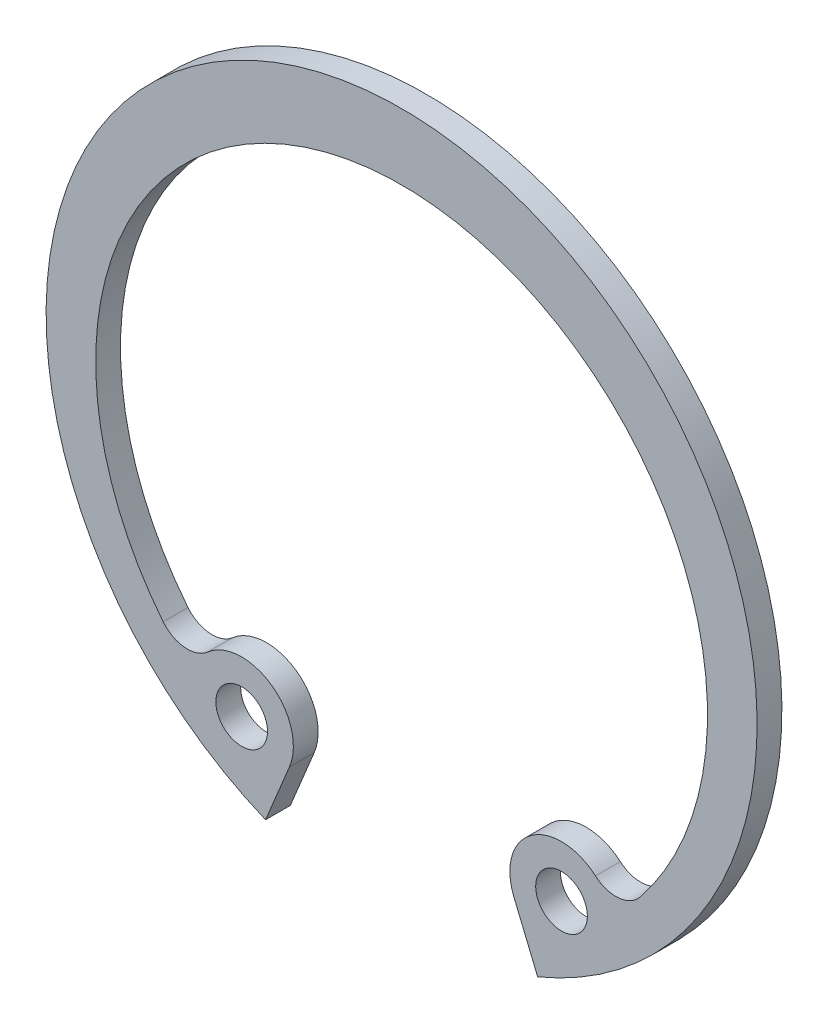
SolidWorks part; units mm, degrees
ref_plane "前视基准面" through (0, 0, 0) normal (0, 0, 1) x (1, 0, 0)
ref_plane "上视基准面" through (0, 0, 0) normal (0, 1, 0) x (1, 0, 0)
ref_plane "右视基准面" through (0, 0, 0) normal (1, 0, 0) x (0, 0, -1)
sketch "草图1" plane through (0, 0, 0) normal (0, 0, 1) x (1, 0, 0)
  line L0 (5.427, -13.1018) -> (6.5822, -15.8907)
  line L1 (-6.5822, -15.8907) -> (-5.427, -13.1018)
  circle A0 centre (-7.7367, -12.1451) radius 1.25
  circle A1 centre (7.7367, -12.1451) radius 1.25
  arc A2 (9.3806, -10.2617) -> (5.427, -13.1018) centre (7.7367, -12.1451) ccw
  arc A3 (6.5822, -15.8907) -> (-6.5822, -15.8907) centre (0, 0) ccw
  arc A4 (-5.427, -13.1018) -> (-9.3806, -10.2617) centre (-7.7367, -12.1451) ccw
  arc A5 (-9.3806, -10.2617) -> (-11.5362, -10.0713) centre (-10.367, -9.1316) cw
  arc A6 (-11.5362, -10.0713) -> (11.5362, -10.0713) centre (0, -0.8) cw
  arc A7 (11.5362, -10.0713) -> (9.3806, -10.2617) centre (10.367, -9.1316) cw
extrude "凸台-拉伸1" add sketch "草图1" against normal blind 1.2
